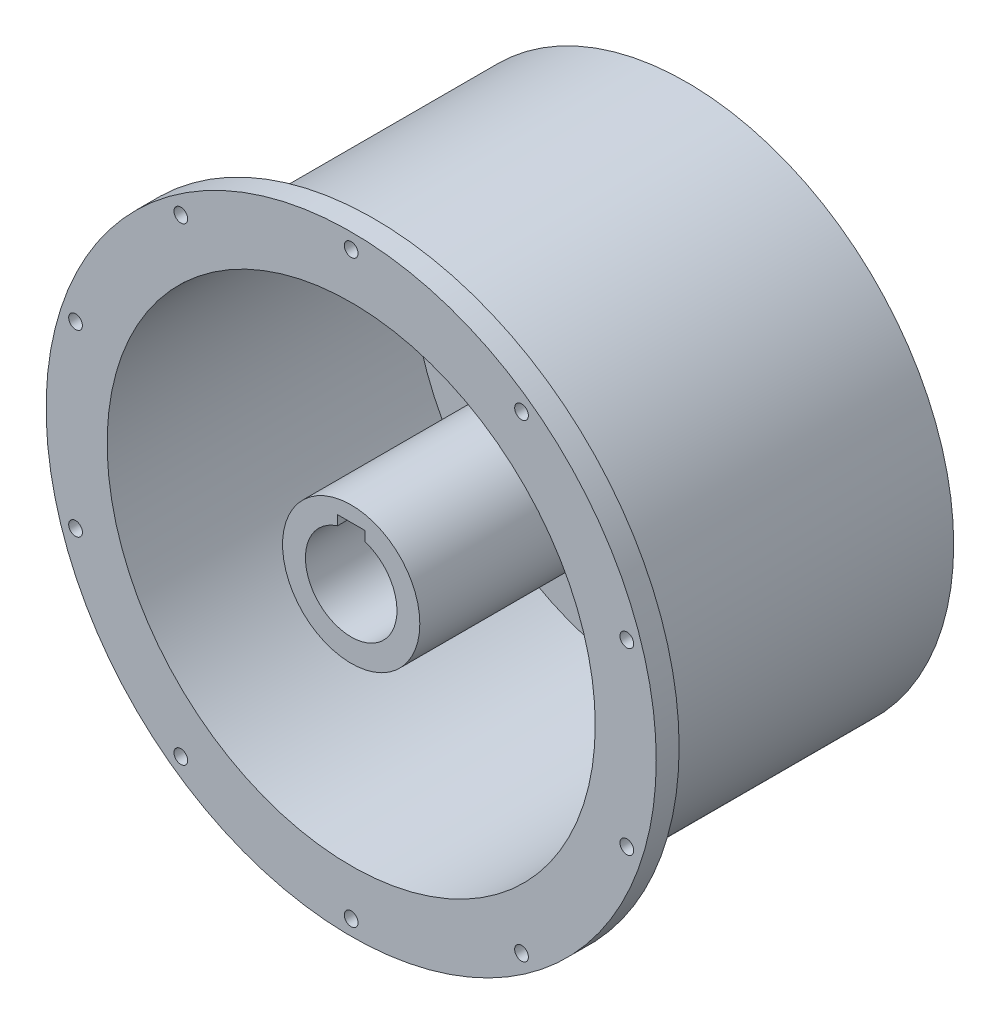
from build123d import *

# Parameters (mm, degrees)
SKETCH1_R           = 175
SKETCH1_R_2         = 30
BOSS_EXTRUDE1_DEPTH = 220
BOSS_EXTRUDE2_START = -15
SKETCH2_R           = 200
SKETCH2_R_2         = 4.5
SKETCH2_R_3         = 30
BOSS_EXTRUDE2_DEPTH = 15
SKETCH3_R           = 160
SKETCH3_R_2         = 45
CUT_EXTRUDE1_DEPTH  = 200
SKETCH4_R           = 30
BOSS_EXTRUDE3_DEPTH = 20
SKETCH7_W           = 18
SKETCH7_H           = 20.211896708
CUT_EXTRUDE2_DEPTH  = 200


with BuildPart() as part:
    # Sketch1 → Boss-Extrude1 (new body)
    with BuildSketch(Plane.XY):
        Circle(SKETCH1_R)
        Circle(SKETCH1_R_2, mode=Mode.SUBTRACT)
    extrude(amount=BOSS_EXTRUDE1_DEPTH)

    # Sketch2 → Boss-Extrude2 (add)
    with BuildSketch(Plane.XY.offset(220).offset(BOSS_EXTRUDE2_START)):
        Circle(SKETCH2_R)
        with Locations((0, 190)):
            Circle(SKETCH2_R_2, mode=Mode.SUBTRACT)
        with Locations((111.679197936, 153.713228931)):
            Circle(SKETCH2_R_2, mode=Mode.SUBTRACT)
        with Locations((180.700738096, 58.713228931)):
            Circle(SKETCH2_R_2, mode=Mode.SUBTRACT)
        with Locations((180.700738096, -58.713228931)):
            Circle(SKETCH2_R_2, mode=Mode.SUBTRACT)
        with Locations((111.679197936, -153.713228931)):
            Circle(SKETCH2_R_2, mode=Mode.SUBTRACT)
        with Locations((0, -190)):
            Circle(SKETCH2_R_2, mode=Mode.SUBTRACT)
        with Locations((-111.679197936, -153.713228931)):
            Circle(SKETCH2_R_2, mode=Mode.SUBTRACT)
        with Locations((-180.700738096, -58.713228931)):
            Circle(SKETCH2_R_2, mode=Mode.SUBTRACT)
        with Locations((-180.700738096, 58.713228931)):
            Circle(SKETCH2_R_2, mode=Mode.SUBTRACT)
        with Locations((-111.679197936, 153.713228931)):
            Circle(SKETCH2_R_2, mode=Mode.SUBTRACT)
        Circle(SKETCH2_R_3, mode=Mode.SUBTRACT)
    extrude(amount=BOSS_EXTRUDE2_DEPTH)

    # Sketch3 → Cut-Extrude1 (cut)
    with BuildSketch(Plane.XY.offset(220)):
        Circle(SKETCH3_R)
        Circle(SKETCH3_R_2, mode=Mode.SUBTRACT)
    extrude(amount=-CUT_EXTRUDE1_DEPTH, mode=Mode.SUBTRACT)

    # Sketch4 → Boss-Extrude3 (add)
    with BuildSketch(Plane(origin=(0, 0, 0), x_dir=(-1, 0, 0), z_dir=(0, 0, -1))):
        Circle(SKETCH4_R)
    extrude(amount=-BOSS_EXTRUDE3_DEPTH)

    # Sketch7 → Cut-Extrude2 (cut)
    with BuildSketch(Plane.XY.offset(220)):
        with Locations((0, 24.894051646)):
            Rectangle(SKETCH7_W, SKETCH7_H)
    extrude(amount=-CUT_EXTRUDE2_DEPTH, mode=Mode.SUBTRACT)


solid = part.part
